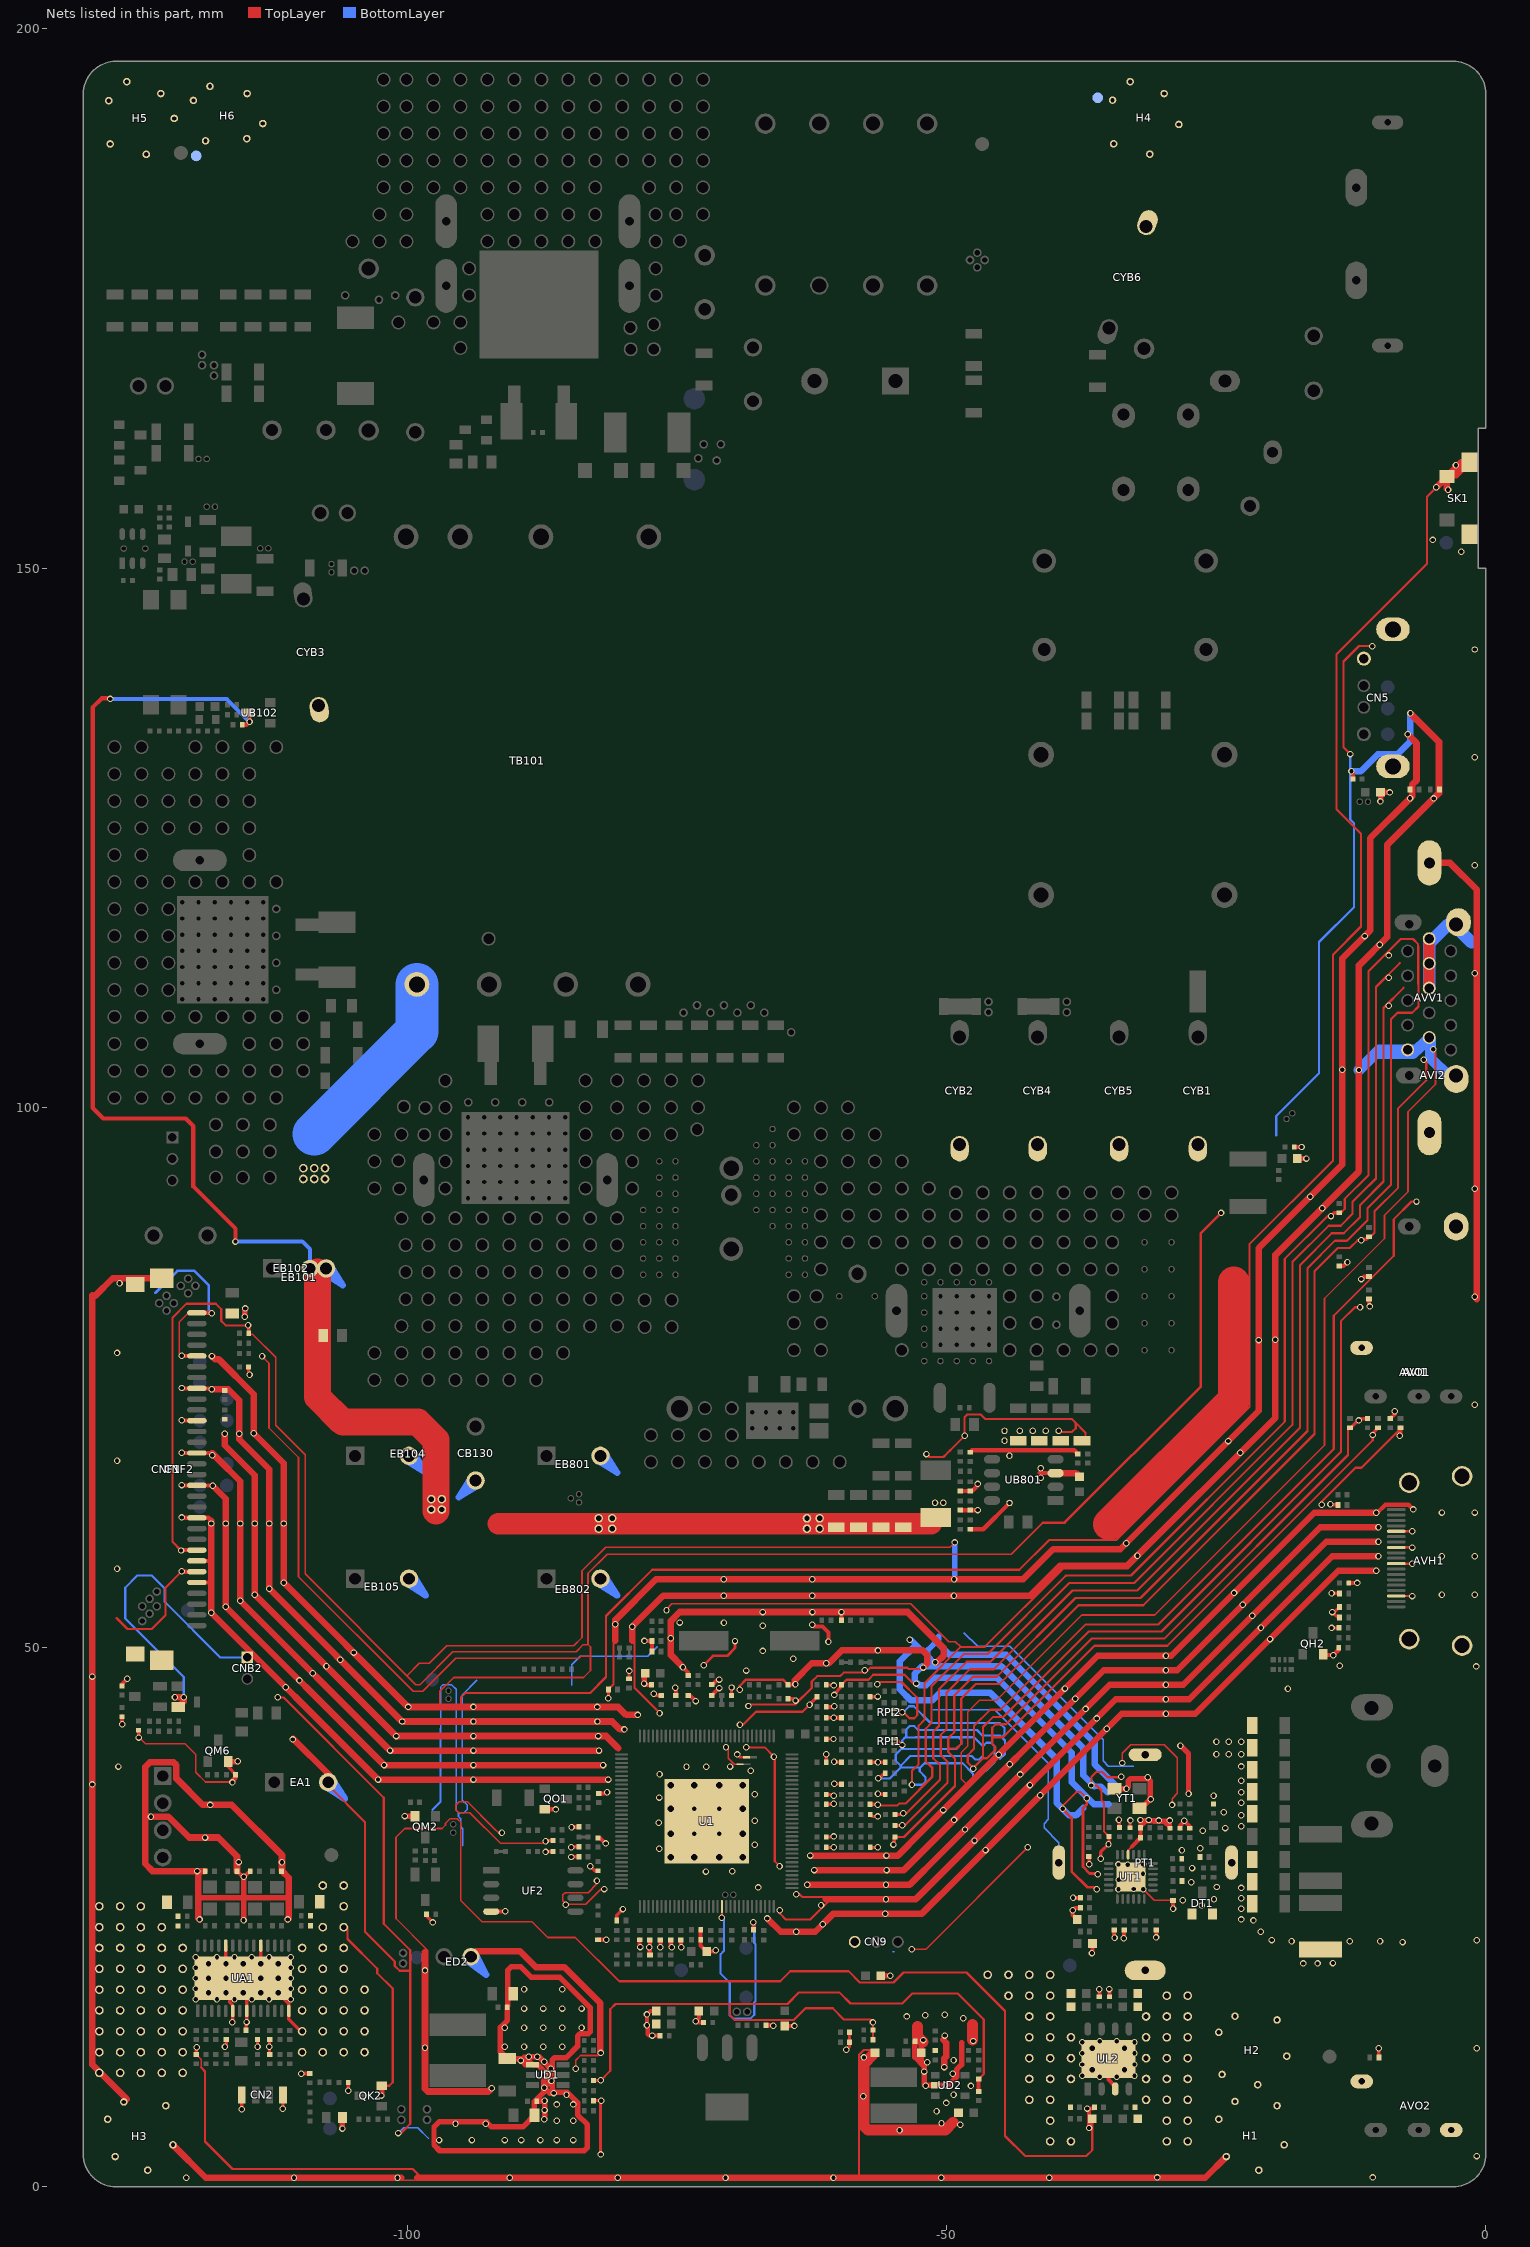
[diagram p0: the nets of this part, all layers, seen from the top]
# Altium PCB MISC84438.PcbDoc (part 9 of 15)
Units mm, origin at the board's own origin, x right, y up, seen from the top; angles counter-clockwise.
Board outline 130 x 197 mm, 2 copper layers (TopLayer, BottomLayer), stack 1.571 mm thick; 574 components, 314 nets, 2636 pads, 811 vias.

## Via types
v1: diameter 0.6, hole 0.4, TopLayer to BottomLayer, tented both sides, 780 vias
v2: diameter 0.7, hole 0.5, TopLayer to BottomLayer, tented both sides, 15 vias
v3: diameter 0.8, hole 0.6, TopLayer to BottomLayer, tented both sides, 12 vias
v4: diameter 0.8, hole 0.5, TopLayer to BottomLayer, tented both sides, 4 vias

## Nets (pads, with @x,y where several pads share a name; then routed paths per layer and width w, separated by ;. In a path a pad name is that pad's centre, name@x,y a point inside that pad or via, vN(x,y) a via of type N, cw(c..) or ccw(c..) an arc to the next point about the centre after c; other vN are vias at no path point) (continued)
GND: AVH1.5 AVH1.8 AVH1.11 AVH1.17 AVH1.20 AVH1.21 AVH1.22 AVH1.23 AVI1.1 AVI2.2 AVI2.4 AVI2.6 AVO1.1 AVO2.1 AVO2.3 AVV1.5 AVV1.6 AVV1.7 AVV1.8 AVV1.10 AVV1.16 AVV1.17 CA4.2 CA5.2 CA10.2 CA15.2 CA16.1 CA17.1 CA18.2 CA23.1 CA24.1 CA25.1 CA28.1 CA31.1 CA32.1 CB130.1 CB131.2 CB801.1 CB803.2 CB804.2 CB805.1 CB806.2 CB812.1 CB813.1 CD1.2 CD11.1 CD12.2 CD14.1 CD15.1 CD16.1 CD17.1 CD19.2 CD21.2 CD22.2 CD41.1 CF1.1 CF2.1 CF4.1 CF5.2 CF6.1 CF7.1 CF8.1 CF9.1 CF10.1 CF12.1 CF13.1 CF14.1 CF15.2 CF16.1 CF17.1 CF18.1 CF19.1 CF20.1 CF21.1 CF22.2 CF23.1 CF24.1 CF25.1 CF29.2 CF30.2 CF33.1 CF35.1 CF37.2 CF38.2 CF39.1 CG1.2 CH8.1 CH9.1 CH10.1 CI10.2 CI11.2 CK2.2 CK4.2 CK6.1 CK10.1 CL1.1 CL2.1 CL3.1 CL4.1 CL5.1 CL6.1 CL7.1 CL8.1 CL9.1 CL10.1 CL11.2 CL12.2 CL13.2 CL14.2 CL15.1 CM2.2 CM4.2 CM5.1 CN2.1 CN2.4 CN5.4 CN5.5 CN5.6 CN9.1 CNB2.1 CNF1.1 CNF1.5 CNF1.8 CNF1.11 CNF1.14 CNF1.17 CNF1.20 CNF1.23 CNF1.24 CNF1.25 CNF1.26 CNF1.31 CNF1.32 CNF2.1 CNF2.5 CNF2.8 CNF2.11 CNF2.14 CNF2.17 CNF2.20 CNF2.23 CNF2.24 CNF2.25 CNF2.26 CNF2.31 CNF2.32 CO3.1 CO5.1 CO9.1 CT1.1 CT3.2 CT5.1 CT6.2 CT7.1 CT8.1 CT9.2 CT10.2 CT11.1 CT12.2 CT14.1 CT15.1 CT17.2 CT18.1 CT19.1 CT21.2 CT24.1 CT25.2 CT26.1 CT27.2 CT29.1 CT41.1 CT42.1 CT43.1 CT44.1 CT45.1 CT46.1 CT47.1 CT48.1 CU1.1 CU2.2 CU3.2 CU4.1 CV9.1 CV10.1 CYB1.2 CYB2.2 CYB3.2 CYB4.2 CYB5.2 CYB6.2 DB804.K DH2.A DH3.A DH6.A DH7.A DH8.A DH9.A DI1.A DI2.A DI3.A DI5.A DK1.A DK20.K DO1.A DO2.A DO3.A DT1.1 DT1.3 DT2.A DT3.A DU1.A DU2.A DU3.A DU4.A DV1.A DV2.A EA1.2 EB101.2 EB102.2 EB104.2 EB105.2 EB801.2 EB802.2 ED2.2 GDT2.1 H1.1@-24.05,2.786 H1.2 H1.3 H1.4 H1.5 H1.6 H2.1@-24.45,10.4 H2.2 H2.3 H2.4 H2.5 H2.6 H3.1@-127.05,2.786 H3.2 H3.3 H3.4 H3.5 H3.6 H4.1@-34.5,189.35 H4.2 H4.3 H4.4 H4.5 H4.6 H5.1@-127.513,189.342 H5.2 H5.3 H5.4 H5.5 H5.6 H6.1@-118.674,189.636 H6.2 H6.3 H6.4 H6.5 H6.6 LF6.1 LT6.2 LT8.2 LT11.2 pad.VIA5@-27.635,4.191 pad.VIA5@-27.635,6.121 pad.VIA5@-27.635,8.052 pad.VIA5@-27.635,9.982 pad.VIA5@-27.635,11.913 pad.VIA5@-27.635,13.843 pad.VIA5@-27.635,15.773 pad.VIA5@-27.635,17.704 pad.VIA5@-29.566,4.191 pad.VIA5@-29.566,6.121 pad.VIA5@-29.566,8.052 pad.VIA5@-29.566,9.982 pad.VIA5@-29.566,11.913 pad.VIA5@-29.566,13.843 pad.VIA5@-29.566,15.773 pad.VIA5@-29.566,17.704 pad.VIA5@-31.496,8.052 pad.VIA5@-31.496,9.982 pad.VIA5@-31.496,11.913 pad.VIA5@-31.496,13.843 pad.VIA5@-31.496,15.773 pad.VIA5@-38.456,4.191 pad.VIA5@-38.456,9.982 pad.VIA5@-38.456,11.913 pad.VIA5@-38.456,13.843 pad.VIA5@-39.599,70.053 pad.VIA5@-40.386,4.191 pad.VIA5@-40.386,6.121 pad.VIA5@-40.386,8.052 pad.VIA5@-40.386,9.982 pad.VIA5@-40.386,11.913 pad.VIA5@-40.386,13.843 pad.VIA5@-40.386,15.773 pad.VIA5@-40.386,17.704 pad.VIA5@-40.386,19.634 pad.VIA5@-40.799,70.053 pad.VIA5@-41.262,65.697 pad.VIA5@-41.262,66.599 pad.VIA5@-41.999,70.053 pad.VIA5@-42.316,8.052 pad.VIA5@-42.316,9.982 pad.VIA5@-42.316,11.913 pad.VIA5@-42.316,13.843 pad.VIA5@-42.316,15.773 pad.VIA5@-42.316,17.704 pad.VIA5@-42.316,19.634 pad.VIA5@-43.199,70.053 pad.VIA5@-44.146,63.372 pad.VIA5@-44.158,67.754 pad.VIA5@-44.247,17.704 pad.VIA5@-44.247,19.634 pad.VIA5@-44.615,69.151 pad.VIA5@-44.615,70.053 pad.VIA5@-46.177,19.634 pad.VIA5@-50.292,63.386 pad.VIA5@-51.054,63.386 pad.VIA5@-61.759,60.985 pad.VIA5@-61.759,61.951 pad.VIA5@-62.928,60.985 pad.VIA5@-62.928,61.951 pad.VIA5@-80.989,60.985 pad.VIA5@-80.989,61.951 pad.VIA5@-82.233,60.985 pad.VIA5@-82.233,61.951 pad.VIA5@-96.774,62.763 pad.VIA5@-96.774,63.729 pad.VIA5@-97.739,62.763 pad.VIA5@-97.739,63.729 pad.VIA5@-103.937,12.471 pad.VIA5@-103.937,14.402 pad.VIA5@-103.937,16.332 pad.VIA5@-103.937,18.263 pad.VIA5@-105.867,12.471 pad.VIA5@-105.867,14.402 pad.VIA5@-105.867,16.332 pad.VIA5@-105.867,18.263 pad.VIA5@-105.867,20.193 pad.VIA5@-105.867,22.123 pad.VIA5@-105.867,24.054 pad.VIA5@-105.867,25.984 pad.VIA5@-105.867,27.915 pad.VIA5@-107.6,93.4 pad.VIA5@-107.6,94.4 pad.VIA5@-107.798,12.471 pad.VIA5@-107.798,14.402 pad.VIA5@-107.798,16.332 pad.VIA5@-107.798,18.263 pad.VIA5@-107.798,20.193 pad.VIA5@-107.798,22.123 pad.VIA5@-107.798,24.054 pad.VIA5@-107.798,27.915 pad.VIA5@-108.6,93.4 pad.VIA5@-108.6,94.4 pad.VIA5@-109.6,93.4 pad.VIA5@-109.6,94.4 pad.VIA5@-109.728,12.471 pad.VIA5@-109.728,14.402 pad.VIA5@-109.728,16.332 pad.VIA5@-109.728,18.263 pad.VIA5@-109.728,20.193 pad.VIA5@-109.728,22.123 pad.VIA5@-120.802,10.541 pad.VIA5@-120.802,12.471 pad.VIA5@-120.802,14.402 pad.VIA5@-120.802,16.332 pad.VIA5@-120.802,18.263 pad.VIA5@-120.802,20.193 pad.VIA5@-120.802,22.123 pad.VIA5@-122.733,10.541 pad.VIA5@-122.733,12.471 pad.VIA5@-122.733,14.402 pad.VIA5@-122.733,16.332 pad.VIA5@-122.733,18.263 pad.VIA5@-122.733,20.193 pad.VIA5@-122.733,22.123 pad.VIA5@-122.733,24.054 pad.VIA5@-124.663,10.541 pad.VIA5@-124.663,12.471 pad.VIA5@-124.663,14.402 pad.VIA5@-124.663,16.332 pad.VIA5@-124.663,18.263 pad.VIA5@-124.663,20.193 pad.VIA5@-124.663,22.123 pad.VIA5@-124.663,24.054 pad.VIA5@-124.663,25.984 pad.VIA5@-126.594,10.541 pad.VIA5@-126.594,12.471 pad.VIA5@-126.594,14.402 pad.VIA5@-126.594,16.332 pad.VIA5@-126.594,18.263 pad.VIA5@-126.594,20.193 pad.VIA5@-126.594,22.123 pad.VIA5@-126.594,24.054 pad.VIA5@-126.594,25.984 pad.VIA5@-128.524,10.541 pad.VIA5@-128.524,12.471 pad.VIA5@-128.524,14.402 pad.VIA5@-128.524,16.332 pad.VIA5@-128.524,18.263 pad.VIA5@-128.524,20.193 pad.VIA5@-128.524,22.123 pad.VIA5@-128.524,24.054 pad.VIA5@-128.524,25.984 PT1.1 PT1.2 PT1.3 PT1.4 QH2.E QK2.E QM2.E QM6.E QO1.E R1.2 R2.2 RA1.1 RA2.JP_2K RA12.2 RA14.1 RA15.JP_2K RB134.1 RB140.2 RB803.1 RB818.2 RB819.2 RB820.2 RB821.2 RB837.1 RB838.1 RB839.2 RB840.1 RD7.1 RD16.1 RD88.1 RF12.2 RF14.1 RF15.1 RF16.2 RF19.1 RF21.1 RF22.1 RH29.2 RI3.1 RI9.1 RL2.2 RL4.1 RM6.2 RM10.2 RO3.1 RO4.1 RO7.1 RO8.1 RO12.2 RPI1.4 RPI1.6 RPI2.4 RPI2.6 RR1.1 RV2.1 RV5.1 RV11.1 RV13.2 RV14.2 SK1.1 SK1.3 SK1.4 TB101.6 TB-GND1.1 TB-GND2.1 U1.116 U1.129 UA1.6 UA1.8 UA1.14 UA1.19 UA1.24 UA1.EPAD@-115.175,19.315 UB102.A UB801.3 UD1.1 UD2.2 UF2.4 UL2.3 UL2.EPAD UT1.10 UT1.25 YT1.2 YT1.4 | length 4276
  TopLayer w0.127: v1(-85.281,26.137) -85.281,26.251 -85.547,26.518 ; v1@-82.396,28.267 v1(-82.396,28.349) -82.396,28.082 -83.215,27.262 -85.336,27.262 -85.547,27.051 -85.547,26.518 ; v1(-81.712,27.584) -82.029,27.584 -83.426,26.187 -85.217,26.187 -85.547,26.518 ; v1(-75.946,53.442) -75.946,53.518 -75.451,54.013 -53.284,54.013 -49.799,50.528 -49.162,50.528 -48.665,50.032 ; -51.477,38.988 -51.423,38.988 -51.288,38.852 -51.288,37.959 -51.325,37.959 -51.333,37.968 ; v1(-33.706,39.268) -33.706,40.169 -32.924,40.951 -29.808,40.951 -28.607,39.75 -28.607,36.443 -29.083,35.966 v1(-29.083,35.382)
  TopLayer w0.152: v1(-124.854,41.631) -124.816,41.631 -124.223,41.038 -120.565,41.038 -119.583,40.056 -119.583,38.401 -118.686,37.503 -116.529,37.503 RM10.2@-115.856,38.176 ; v1(-120.886,77.029) -121.11,77.253 -121.11,80.152 -120.262,81 CNF2.1@-119.486,81 ; RA1.1@-119.544,12.247 -119.083,11.785 -119.083,11.044 ; RF21.1@-114.656,79.019 -114.314,79.019 -112.18,76.885 -112.18,70.579 -109.442,67.841 -109.442,56.799 -99.176,46.533 -98.796,46.533 -95.748,49.581 -84.316,49.581 -83.681,50.216 -83.223,50.216 ; v1(-113.439,76.966) -112.79,76.316 -112.79,70.327 -110.051,67.588 -110.051,56.546 -99.428,45.923 -98.543,45.923 -95.495,48.971 -84.049,48.971 -83.841,49.179 -83.071,49.179 ; v1@-100.851,0.826 -100.622,0.597 -99.276,0.597 -99.047,0.826 ; -99.987,47.371 -98.857,48.501 -97.942,48.501 -96.304,50.14 -84.547,50.14 -83.782,50.905 -83.782,57.077 -81.59,59.268 -49.675,59.268 v1(-49.233,59.71) ; -98.065,16.751 -98.065,21.897 -101.016,24.848 -101.016,32.396 -100.214,33.198 -96.761,33.198 -96.431,33.528 -96.431,33.688 -96.014,34.104 -95.352,34.104 -95.004,33.757 -95.004,26.499 -93.054,24.549 -88.406,24.549 -86.95,23.093 -84.398,23.093 -80.329,19.024 ; -96.952,44.539 -96.952,45.906 -95.664,47.193 -83.642,47.193 -82.995,47.841 -82.995,50.025 -83.223,50.254 -83.223,56.845 -81.445,58.623 -43.984,58.623 -41.063,61.544 ; -91.55,32.829 -91.952,33.232 ; v1(-91.198,32.794) -91.515,32.794 -91.952,33.232 ; v1(-87.16,32.029) -87.363,31.826 -91.337,31.826 -94.174,34.663 -95.204,34.663 -95.485,34.944 -95.485,35.357 -95.168,35.674 -94.394,35.674 -91.952,33.232 ; v1(-84.366,10.935) -84.366,11.71 -83.926,12.15 -82.287,12.15 v1(-82.042,12.395) ; v1(-70.432,40.718) -70.348,40.718 -70.232,40.602 -70.232,39.719 -69.679,39.167 RA15.JP_2K@-69.129,39.167 ; v1@-54.225,41.025 v1@-54.14,41.11 ; v1(-53.2,22) -51.899,22 v1(-42.451,31.448) ; -48.184,37.351 -48.616,37.782 -48.616,40.235 -48.038,40.813 -48.038,43.967 -46.932,45.072 -45.362,45.072 -37.45,52.984 -30.703,52.984 -14.961,68.727 -14.961,82.325 -9.398,87.888 -9.398,90.04 -7.214,92.224 -7.214,99.642 -4.662,102.194 -4.662,105.21 v1(-4.886,105.434) ; UT1.25@-32.906,28.714 -30.728,26.537 LT6.2@-28.981,26.537
  TopLayer w0.191: v1(-70.815,24.915) -70.812,24.918 U1.116@-70.812,25.971 ; UT1.25@-33.156,28.964 UT1.25@-32.906,28.714 ; UT1.10@-33.156,30.764 -33.156,31.182 -32.798,31.54
  TopLayer w0.2: v1(-51.854,67.907) -51.574,67.627 -50.278,67.627 -49.885,68.02 ; -49.619,68.286 -49.885,68.02 ; pad.VIA5@-39.599,70.053 -39.491,69.945 -38.371,69.945 -38.018,70.299 -38.018,70.798 -38.118,70.899 ; -37.109,69.672 -37.109,69.89 -38.118,70.899 ; -49.885,68.02 v1(-48.311,69.594) -48.311,71.349 -48.082,71.577 -46.812,71.577 -46.395,71.16 -38.964,71.16 -38.379,71.16 -38.118,70.899
  TopLayer w0.203: -126.924,52.705 -125.908,51.689 -123.675,51.689 -122.395,52.969 -122.395,55.521 v1(-120.886,57.029) ; v1@-120.913,59 v1(-120.947,58.966) -121.745,59.764 -121.745,80.535 -120.45,81.829 -117.715,81.829 -117.227,81.342 -117.227,80.244 -116.815,79.832 v1(-114.732,79.832) ; -119.083,11.044 -118.72,10.681 -118.72,4.177 -116.181,1.638 -99.454,1.638 -98.857,1.041 -97.904,1.041 ; v1@-118.102,67.793 -117.583,67.793 ; v1(-111.976,45.352) -111.454,45.352 -102.159,36.057 -102.159,24.374 -99.704,21.92 -99.704,5.818 -100.557,4.966 v1(-100.813,4.966) ; EA1.2@-107.304,37.207 -103.886,33.789 -103.886,23.628 -101.13,20.872 -101.13,20.46 -100.686,20.015 -99.784,20.015 ; pad.VIA5@-105.512,24.105 -105.512,22.954 -102.756,20.198 -102.756,19.786 -101.33,18.36 -101.33,9.665 -101.635,9.36 QK2.E@-102.349,9.36 ; -94.983,44.704 -94.983,45.364 -94.602,45.745 -83.042,45.745 -81.547,47.241 -81.547,52.892 -77.263,57.175 -43.24,57.175 -40.471,59.944 -34.248,59.944 -21.92,72.272 -21.92,87.359 -14.173,95.106 -14.173,114.198 -11.57,116.802 -11.57,125.412 -13.856,127.698 -13.856,142.024 -5.447,150.433 -5.447,156.656 SK1.1@-3.603,158.5 ; UF2.4@-92.862,25.502 UF2.4@-92.19,25.502 ; v1@-82.055,9.842 -81.153,10.744 -81.153,16.451 -80.67,16.934 -64.737,16.934 -63.666,18.006 -59.925,18.006 -58.893,16.974 -54.088,16.974 -53.161,17.901 -48.951,17.901 -46.537,15.486 -46.537,10.442 RD7.1@-47.015,9.964 ; DU1.A@-81.324,46.101 -80.861,46.564 -80.861,50.622 ; -80.785,50.495 -80.683,50.597 ; -80.311,19.042 -65.395,19.042 -64.476,19.962 -59.064,19.962 -58.032,18.929 -54.898,18.929 -53.971,19.856 -48.141,19.856 -44.564,16.279 -44.564,4.691 -42.705,2.832 -37.033,2.832 -36.482,3.383 CL7.1@-36.482,6.299 ; -79.134,50.622 -78.912,50.4 -78.912,46.249 -76.588,43.925 v1(-76.588,43.876) ; U1.129@-72.212,33.871 U1.129@-71.323,33.871 ; -70.06,16.815 -70.06,15.898 -69.622,15.461 -66.904,15.461 -64.127,15.461 -63.055,16.533 -60.536,16.533 -59.503,15.5 -57.09,15.5 v1(-56.81,15.22) ; v1(-69.399,40.064) -69.399,40.037 -69.163,39.802 RA2.JP_2K@-68.543,39.802 ; v1(-69.14,42.823) -68.861,42.823 -67.659,44.024 -63.341,44.024 v1(-62.687,44.678) ; v1@-68.553,40.627 v1(-68.553,40.716) ; v1(-68.351,44.552) -68.218,44.685 -64.027,44.685 -62.484,46.228 -62.484,46.816 -61.98,47.32 -59.855,47.32 -59.529,47.646 -57.504,47.646 -57.049,48.101 ; -67.029,40.716 v1(-68.553,40.716) ; v1@-65.467,29.794 v1(-65.467,29.705) -65.913,30.151 -65.913,39.727 -65.888,39.752 v1(-65.988,39.853) -66.851,40.716 v1(-68.553,40.716) ; v1(-65.458,25.611) -65.458,25.33 -64.89,24.762 -62.624,24.762 -60.735,26.651 ; v1(-63.932,27.099) -63.614,27.099 -63.369,26.855 -61.326,26.855 ; v1@-60.453,44.475 v1(-60.411,44.516) ; RO7.1@-59.734,46.507 -59.255,46.986 -57.23,46.986 -56.775,47.441 -53.877,47.441 -53.07,46.634 v1(-52.794,46.634) ; -58.102,1.143 -58.102,12.236 -57.664,12.675 CD15.1@-56.545,12.675 ; v1(-57.582,47.854) -57.297,47.854 -57.049,48.101 ; v1(-56.81,15.22) v1(-56.81,15.22) ; RF14.1@-56.808,13.53 RF14.1@-56.808,13.602 v1(-56.81,15.22) ; CF29.2@-56.808,14.516 CF29.2@-56.808,14.593 ; v1@-56.464,35.433 -56.371,35.34 -54.549,35.34 -54.385,35.504 -53.797,35.504 -51.333,37.968 -51.333,38.844 -51.918,39.428 -51.918,42.452 -51.378,42.992 -51.378,46.385 -48.405,49.359 -46.194,49.359 -38.931,56.622 ; v1(-56.403,46.573) -56.403,46.623 -56.246,46.78 -54.166,46.78 -52.699,45.313 -52.699,43.707 -52.988,43.418 -53.42,43.418 -53.97,43.967 v1(-54.102,43.967) ; v1(-54.91,31.708) v1@-54.864,31.754 ; RV11.1@-54.864,32.328 RV11.1@-54.782,32.41 -53.927,32.41 -49.2,37.138 -49.2,39.674 -49.822,40.296 -49.822,41.584 -49.282,42.124 -49.282,45.517 -47.537,47.263 -45.326,47.263 -38.03,54.559 -32.018,54.559 -16.535,70.042 -16.535,85.13 -13.992,87.673 -12.875,87.673 -10.973,89.575 -10.973,90.692 -8.788,92.877 -8.788,108.217 -8.191,108.814 -6.833,108.814 -6.248,109.398 -6.248,114.922 ; RPI1.6@-54.846,41.025 v1@-54.225,41.025 ; RPI1.4@-54.846,41.525 -54.618,41.525 -54.204,41.11 v1@-54.14,41.11 ; RPI2.6@-54.846,43.743 -54.327,43.743 v1(-54.102,43.967) ; RPI2.4@-54.846,44.243 -54.339,44.243 -54.102,44.005 v1(-54.102,43.967) ; v1(-54.013,34.608) -53.706,34.608 -50.597,37.716 -50.597,39.095 -51.219,39.718 -51.219,42.163 -50.679,42.703 -50.679,46.096 -48.115,48.66 -45.905,48.66 -38.609,55.956 -32.597,55.956 -17.932,70.621 -17.932,85.708 -14.571,89.07 -13.453,89.07 -12.37,90.153 -12.37,91.271 -11.582,92.059 -10.185,93.455 -10.185,111.201 -7.976,113.411 ; v1@-53.849,33.476 -49.898,37.427 -49.898,39.385 -50.521,40.007 -50.521,41.874 -49.981,42.413 -49.981,45.807 -47.826,47.962 -45.615,47.962 -38.319,55.258 -32.308,55.258 -17.234,70.332 -17.234,85.419 -14.281,88.371 -13.164,88.371 -11.671,89.864 -11.671,90.981 -9.487,93.166 -9.487,109.258 -7.62,111.125 ; v1(-53.196,37.247) -53.192,37.251 -53.192,38.552 -52.578,39.167 -52.578,42.726 -52.038,43.265 -52.038,46.659 -48.665,50.032 -46.455,50.032 -39.201,57.286 ; v1@-52.142,47.993 -53.495,47.993 -53.603,48.101 -57.049,48.101 ; -49.784,40.607 -49.07,40.607 -48.622,41.055 -48.622,45.244 -47.263,46.603 -45.053,46.603 -37.756,53.899 -31.745,53.899 -15.875,69.769 -15.875,84.856 -13.719,87.013 -12.601,87.013 -11.882,87.732 v1(-11.557,87.732) v1@-11.481,87.808 ; v1(-47.514,38.727) v1@-47.514,38.8 ; -46.607,42.431 -46.607,42.609 ; -45.745,41.664 -44.747,41.664 -36.271,50.14 -29.525,50.14 -10.49,69.174 v1(-10.49,69.672) ; v1(-39.23,35.027) -39.23,35.309 -37.968,36.571 -37.557,36.571 v1(-37,36.014) ; -38.898,56.655 -32.886,56.655 -18.631,70.91 -18.631,85.998 -14.662,89.967 v1(-14.351,89.967) ; CT14.1@-34.925,32.455 -35.403,32.933 -35.403,35.6 -35.624,35.821 -35.624,36.728 -36.081,37.186 v1(-36.563,37.186) -36.558,37.19 -36.558,37.981 -36.095,38.444 -35.577,38.444 -35.073,37.94 -33.853,37.94 v1(-33.807,37.986) ; v1(-15.215,63.221) -15.215,63.516 -12.088,66.643 -11.526,66.643 -7.899,70.269 DO3.A@-7.899,70.339 ; DI3.A@-13.462,90.246 -13.068,90.64 -13.068,91.56 -10.884,93.745 -10.884,112.662 -7.899,115.646 -6.756,115.646 -6.274,115.164 -6.274,111.481 ; -13.195,139.745 -13.195,139.344 ; DO2.A@-12.573,70.339 -12.776,70.136 -12.776,67.822 -29.798,50.8 -36.545,50.8 -44.484,42.861 -45.421,42.861 -45.745,42.537 -45.745,41.032 -45.466,40.753 -45.466,40.476 -46.235,39.707 -46.607,39.707 ; v1(-12.573,132.791) -13.195,133.413 -13.195,139.344 ; v1(-11.659,81.509) -12.131,81.509 -13.437,80.203 -13.437,68.095 -30.072,51.46 -36.818,51.46 -44.757,43.521 -45.695,43.521 -46.607,42.609 ; DI2.A@-10.668,88.062 -10.312,88.417 -10.312,90.419 -8.128,92.603 -8.128,99.949 -5.526,102.551 -5.526,104.23 v1(-5.74,104.445) ; v1(-10.541,142.799) -11.76,142.799 -13.195,141.364 -13.195,139.344 ; v1(-6.426,91.313) -6.883,91.313 -8.534,89.662 -8.534,86.284 -14.097,80.721 -14.097,68.369 -30.345,52.121 -37.092,52.121 -45.004,44.209 -45.941,44.209 -47.454,42.697 -47.454,40.571 -48.031,39.993 -48.031,39.317 v1@-47.514,38.8 ; v1@-47.514,38.8 -46.607,39.707 ; -46.607,39.707 -46.607,42.609
  TopLayer w0.229: v1(-69.156,46.055) -69.156,46.417 -68.575,46.998 -65.148,46.998 CT24.1@-64.657,46.507 ; AVH1.17@-8.3,54.75 v1@-6.815,54.75 ; AVH1.11@-8.3,57.75 -6.825,57.75 v1(-6.815,57.74) ; AVH1.8@-8.3,59.25 -6.825,59.25 v1(-6.815,59.24) ; AVH1.5@-8.3,60.75 -6.825,60.75 v1(-6.815,60.74) ; v1@-6.825,54.75 v1(-6.815,54.74)
  TopLayer w0.254: v1(-72.504,48.323) -71.628,49.2 -70.318,49.2 -69.596,49.922 v1(-69.596,50.571) ; -41.063,61.544 -39.057,61.544 -26.416,74.185 -26.416,88.382 v1(-24.541,90.256) ; v1(-39.23,35.027) -38.392,34.188 -38.392,29.231 -36.911,27.749 -36.233,27.749 v1(-36.055,27.572) ; v1(-37,36.014) -37,35.428 -37.351,35.077 -37.351,29.662 -36.721,29.032 -36.027,29.032 v1(-35.958,28.964)
  TopLayer w0.305: RM6.2@-124.892,42.31 -124.854,42.272 v1(-124.854,41.631) ; RA1.1@-119.544,12.247 -119.544,12.866 v1(-119.482,12.929) ; v1(-116.877,12.954) -116.737,13.094 RA14.1@-116.737,13.632 ; UA1.24@-116.8,22.34 -116.8,20.94 v2(-115.175,19.315) ; QM6.E@-116.573,39.395 -116.573,38.913 RM10.2@-115.856,38.196 ; v1(-116.192,15.24) -116.15,15.282 UA1.6@-116.15,16.29 -116.15,16.798 -116.434,17.081 -116.434,18.056 v2(-115.175,19.315) ; -115.882,37.852 RM10.2@-115.882,38.176 ; v1(-115.316,7.188) -115.305,7.199 CN2.1@-115.305,8.502 ; CA28.1@-114.916,14.503 -114.916,15.208 v1(-114.871,15.253) -114.85,15.274 UA1.8@-114.85,16.29 -114.85,18.99 v2(-115.175,19.315) ; v1(-114.732,79.832) -114.668,79.768 RF21.1@-114.668,79.109 ; RF22.1@-114.693,75.972 -114.693,75.368 v1(-114.595,75.269) ; v1(-113.855,12.954) -113.854,12.955 CA15.2@-113.854,13.632 ; UA1.19@-113.55,22.34 -113.55,20.939 v2(-115.175,19.315) ; RA12.2@-112.737,12.247 -112.737,12.915 v1(-112.776,12.954) -112.737,12.993 CA18.2@-112.737,13.632 ; v1(-111.506,7.214) -111.495,7.225 CN2.4@-111.495,8.502 ; pad.VIA5@-109.728,14.402 -109.855,14.402 -110.95,15.497 UA1.14@-110.95,16.29 -110.95,16.97 -113.295,19.315 v2(-115.175,19.315) ; v1(-105.461,8.903) -105.442,8.921 CK10.1@-105.442,9.652 ; CM2.2@-98.19,25.248 -98.19,25.076 v1(-97.599,24.486) ; v1(-87.16,32.029) -87.109,32.08 CG1.2@-86.48,32.08 ; v1(-87.158,31.023) -87.116,31.064 CF2.1@-86.48,31.064 ; v1(-84.785,30.556) -84.76,30.582 RR1.1@-84.067,30.582 ; v1(-84.785,31.445) -84.734,31.496 CK6.1@-84.067,31.496 ; v1(-83.007,29.693) -82.595,29.28 CF20.1@-82.296,29.28 ; RD88.1@-82.721,7.977 -82.005,7.977 v1(-81.991,7.963) -82.055,7.899 v1(-82.055,2.984) ; RD16.1@-82.721,9.842 -82.055,9.842 v1(-82.029,9.868) ; v1(-81.356,45.263) -81.324,45.295 DU1.A@-81.324,46.101 ; DH8.A@-80.562,24.689 -80.562,25.153 v1(-79.985,25.73) ; DU2.A@-79.426,47.085 -79.426,47.777 v1(-79.4,47.803) ; v1(-77.131,45.682) -76.984,45.535 CF9.1@-76.429,45.535 ; CF14.1@-69.926,45.535 -69.926,46.253 v1(-69.913,46.266) ; CT10.2@-64.682,45.212 -64.135,45.212 v1(-63.983,45.059) ; CT24.1@-64.682,46.507 -64.047,46.507 v1(-63.995,46.558) v1@-63.995,46.777 ; v1(-62.687,44.678) -62.687,44.723 RO8.1@-61.995,45.416 ; v1(-61.151,40.069) -61.145,40.063 CF13.1@-61.145,39.344 ; CF8.1@-61.145,31.445 v1@-60.452,31.445 ; CV9.1@-61.145,32.41 -60.503,32.41 v1(-60.452,32.461) ; CV10.1@-61.145,35.433 -60.528,35.433 v1@-60.452,35.357 ; CF10.1@-61.145,36.347 -60.554,36.347 v1(-60.452,36.246) ; LF6.1@-61.145,41.493 v1(-60.467,41.493) ; CO3.1@-61.145,43.459 v1@-60.452,43.459 ; CT19.1@-61.145,46.507 -60.502,46.507 v1(-60.452,46.456) ; v1@-60.528,36.119 v1@-60.452,36.119 ; v1(-60.414,39.395) -60.363,39.344 RO12.2@-59.734,39.344 ; v1(-60.411,37.354) -60.37,37.313 RF19.1@-59.734,37.313 ; v1@-60.401,45.584 v1(-60.411,45.573) -60.411,45.659 -59.734,46.336 RO7.1@-59.734,46.507 ; v1(-59.294,12.695) -59.289,12.695 -58.98,13.004 CF30.2@-58.98,13.398 RF15.1@-58.98,14.313 ; RV14.2@-57.081,35.433 -56.464,35.433 v1@-56.388,35.509 ; CO9.1@-57.081,39.344 v1(-56.35,39.345) RF12.2@-55.67,39.345 ; RO3.1@-57.081,45.416 -56.375,45.416 v1(-56.363,45.428) ; RV13.2@-57.055,31.445 v1(-56.363,31.445) ; RV2.1@-57.055,34.493 -56.879,34.317 v1(-56.378,34.317) ; v1@-56.347,36.515 -56.2,36.368 -55.691,36.368 RI3.1@-55.67,36.347 ; v1(-56.325,37.841) -56.228,37.841 -55.766,38.303 RI9.1@-55.67,38.303 ; v1@-54.839,31.754 RV11.1@-54.839,32.328 ; RV5.1@-54.782,33.476 -54.13,33.476 v1(-54.105,33.501) ; RF16.2@-54.782,34.493 -54.128,34.493 v1(-54.013,34.608) ; CT1.1@-36.805,30.588 -36.767,30.55 v1(-36.767,29.87) ; v1(-35.7,30.4) -35.7,31.026 v1(-34.976,31.75) -34.925,31.801 CT14.1@-34.925,32.455 ; v1(-34.011,34.011) -33.985,33.985 -33.985,33.305 CT15.1@-33.96,33.279 ; CT27.2@-32.982,33.267 -32.982,33.909 v1(-32.944,33.947) ; v1@-14.402,63.144 -14.351,63.195 DH2.A@-13.709,63.195 ; v1(-14.351,89.967) -14.039,90.278 DI3.A@-13.589,90.278 ; v1(-14.3,51.791) CH8.1@-13.608,51.791 ; v1@-14.3,54.991 DH3.A@-13.557,54.991 ; DH7.A@-13.557,52.756 -13.716,52.756 v1(-14.224,53.264) -14.039,53.264 DH6.A@-13.557,53.746 ; DO2.A@-12.573,70.339 -12.528,70.339 v1@-11.836,71.031 ; v1@-11.836,71.145 v1@-11.836,71.031 ; v1@-11.481,87.808 -11.056,87.808 DI2.A@-10.82,88.043 ; CI10.2@-10.973,71.189 -11.678,71.189 v1@-11.836,71.031 ; v1(-10.49,69.672) -10.49,69.825 -10.008,70.307 DO1.A@-10.008,70.339 ; v1(-9.931,12.827) -9.913,12.808 DI5.A@-9.913,11.989